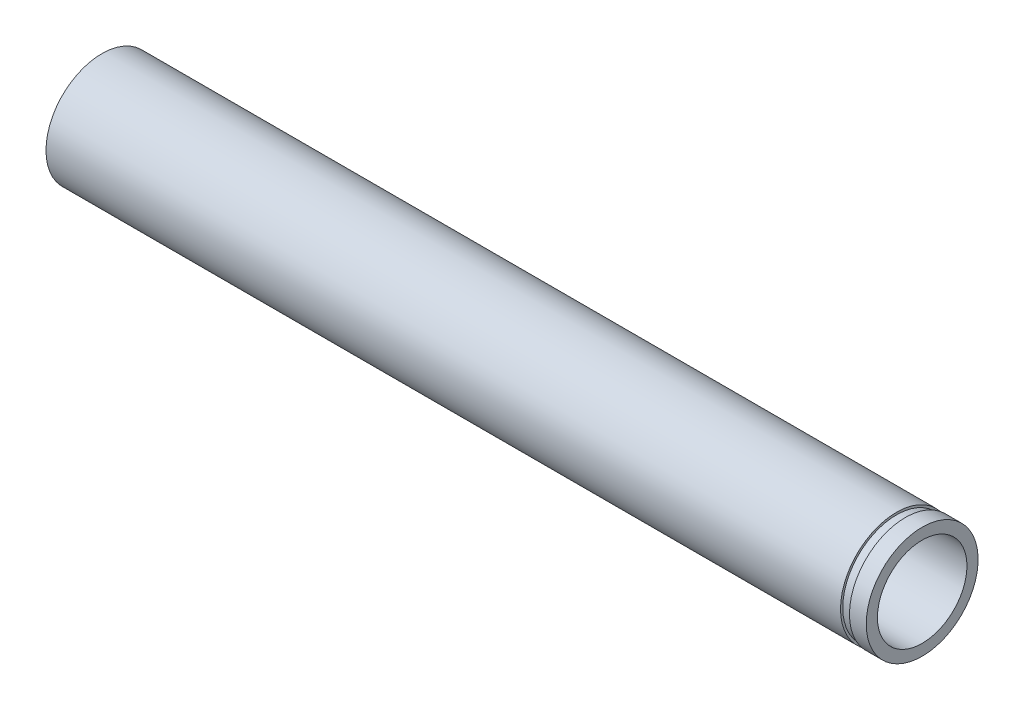
SolidWorks part; units mm, degrees
ref_plane "前视基准面" through (0, 0, 0) normal (0, 0, 1) x (1, 0, 0)
ref_plane "上视基准面" through (0, 0, 0) normal (0, 1, 0) x (1, 0, 0)
ref_plane "右视基准面" through (0, 0, 0) normal (1, 0, 0) x (0, 0, -1)
sketch "草图2" plane through (0, 0, 0) normal (0, 0, 1) x (1, 0, 0)
  line L0 (-27.2143, 0) -> (28.0714, 0) construction
  line L1 (-22.3571, 40) -> (532.6429, 40)
  line L2 (532.6429, 40) -> (532.6429, 50)
  line L3 (532.6429, 50) -> (517.6429, 50)
  line L4 (517.6429, 50) -> (517.6429, 48)
  line L5 (517.6429, 48) -> (509.6429, 48)
  line L6 (509.6429, 48) -> (509.6429, 50)
  line L7 (509.6429, 50) -> (-0.6171, 50)
  line L8 (-0.6171, 50) -> (-0.6171, 48)
  line L9 (-0.6171, 48) -> (-8.6171, 48)
  line L10 (-8.6171, 48) -> (-8.6171, 50)
  line L11 (-8.6171, 50) -> (-22.3571, 50)
  line L12 (-22.3571, 50) -> (-22.3571, 40)
  dimension "D1" = 2
  dimension "D2" = 2
  dimension "D3" = 2
  dimension "D4" = 2
  dimension "D5" = 8
  dimension "D6" = 8
  dimension "D7" = 555
  dimension "D8" = 13.74
  dimension "D9" = 10
  dimension "D10" = 15
  dimension "D11" = 40
revolve "旋转1" add sketch "草图2" angle 360 about L0
sketch "草图3" plane through (-0.6171, 0, 0) normal (-1, 0, 0) x (0, 0, 1)
  circle A0 centre (0, 0) radius 50 construction
  circle A1 centre (0, 0) radius 50
  circle A2 centre (0, 0) radius 40
  dimension "D1" = 80
extrude "凸台-拉伸1" add sketch "草图3" along normal blind 200
sketch "草图4" plane through (-200.6171, 0, 0) normal (-1, 0, 0) x (0, 0, 1)
  circle A0 centre (0, 0) radius 25
  circle A1 centre (0, 0) radius 40 construction
  circle A2 centre (0, 0) radius 40
  dimension "D1" = 50
extrude "凸台-拉伸2" add sketch "草图4" against normal blind 8
